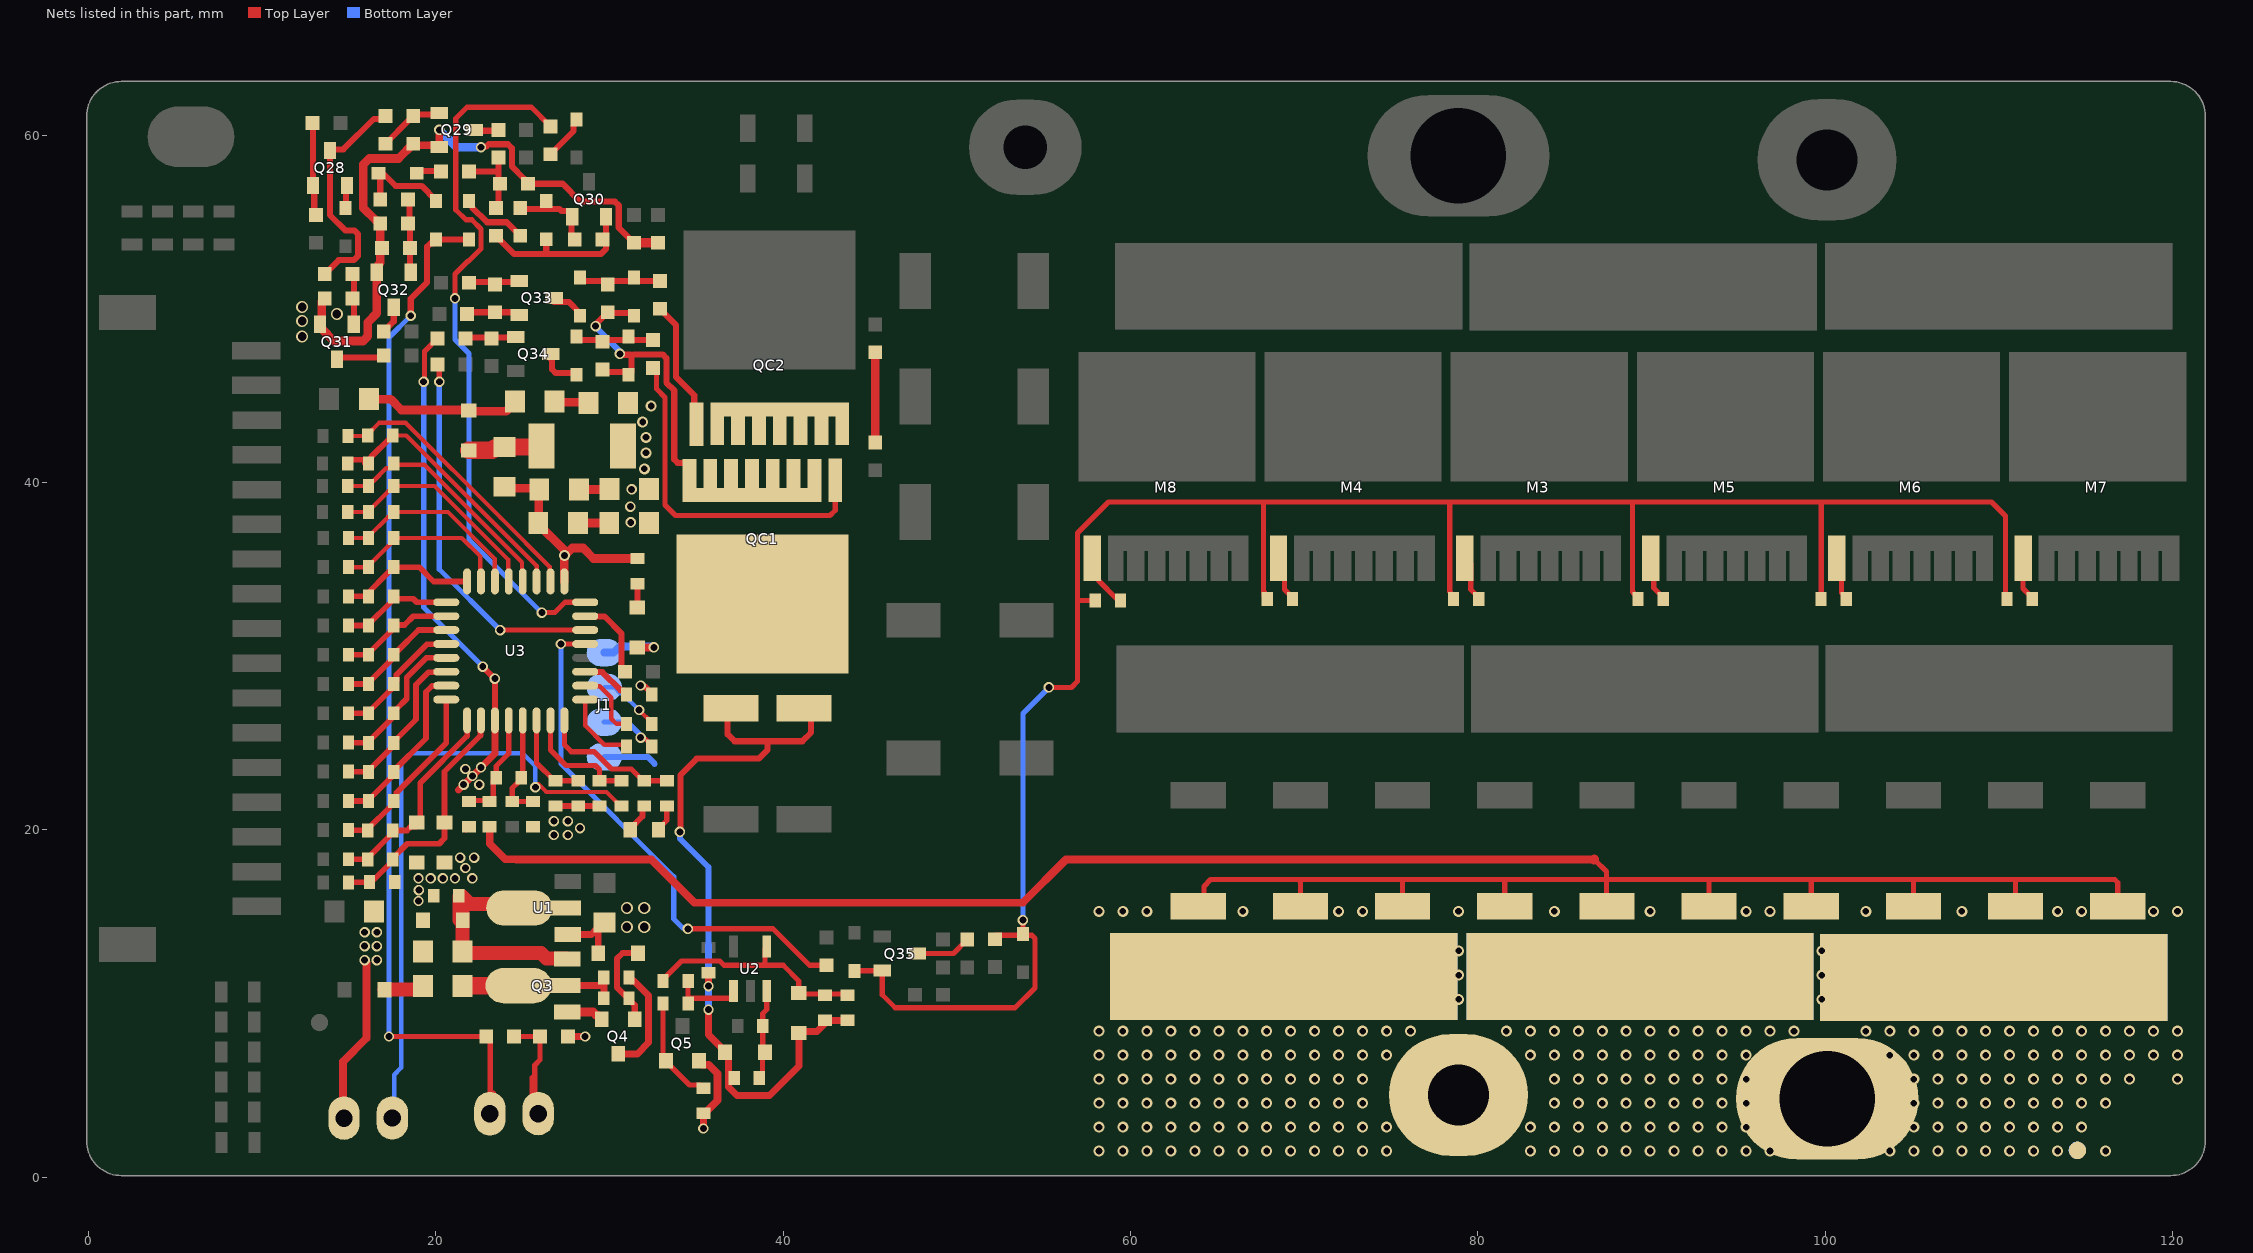
[diagram p0: the nets of this part, all layers, seen from the top]
# Altium PCB MISC86327.PcbDoc (part 2 of 2)
Units mm, origin at the board's own origin, x right, y up, seen from the top; angles counter-clockwise.
Board outline 122 x 63 mm, 2 copper layers (Top Layer, Bottom Layer); 198 components, 117 nets, 551 pads, 998 vias.
Unrouted connection lines stored in the file: 65.

## Via types
v1: diameter 0.635, hole 0.381, Top Layer to Bottom Layer, tented both sides, 846 vias
v2: diameter 0.6, hole 0.4, Top Layer to Bottom Layer, tented both sides, 133 vias
v3: diameter 0.635, hole 0.4, Top Layer to Bottom Layer, tented both sides, 11 vias
v4: diameter 0.7, hole 0.5, Top Layer to Bottom Layer, tented both sides, 8 vias

## Nets (pads, with @x,y where several pads share a name; then routed paths per layer and width w, separated by ;. In a path a pad name is that pad's centre, name@x,y a point inside that pad or via, vN(x,y) a via of type N, cw(c..) or ccw(c..) an arc to the next point about the centre after c; other vN are vias at no path point) (continued)
GND: C2.2 C3.2 C4.2 C6.1 C11.2 C16.2 C25.2 C34.1 C35.1 C36.1 C37.2 C40.2 C41.2 C51.1 C52.1 C53.1 D7.A D8.A D10.A D19.A D20.A J1.4 pad.28@114.522,1.542 pad.29 pad.30@78.88,4.73 pad.30@100.11,4.51 pad.31@68.82,11.55 pad.31@89.33,11.55 pad.31@109.7,11.5 pad.32@68.82,11.55 pad.32@89.33,11.55 pad.32@109.7,11.5 Q5.E Q29.E Q31.E Q32.E R16.1 R76.2 R87.1 R93.1 R126.1 R130.1 R139.1 R140.2 R141.1 R150.2 RN1.1 RN2.1 RN3.1 RN4.1 RN5.1 RN6.1 RN7.1 RN8.1 RN9.1 RN10.1 RT1.2 RT2.2 U1.1 U3.19 | length 233.8
  Top Layer w0.3: v2(19.3,45.8) 19.35,45.85 19.35,46.8 19.35,47.55 R150.2@20.1,48.3 ; RN10.1@63.9,15.602 64.223,15.925 64.223,16.74 64.613,17.13 69.67,17.13 ; RN9.1@69.783,15.602 69.783,17.017 69.67,17.13 ; RN8.1@75.666,15.602 75.666,17.126 75.67,17.13 ; RN7.1@81.549,15.602 81.549,17.116 81.535,17.13 ; 86.69,18.3 87.4,17.59 87.4,17.13 ; RN6.1@87.432,15.602 87.4,15.634 87.4,17.13 ; RN5.1@93.315,15.602 93.315,17.085 93.27,17.13 ; RN4.1@99.198,15.602 99.198,17.092 99.16,17.13 ; RN3.1@105.081,15.602 105.081,17.079 105.03,17.13 ; RN2.1@110.964,15.602 110.964,17.017 110.851,17.13 ; RN1.1@116.847,15.602 116.847,16.954 116.671,17.13 110.851,17.13 ; 69.67,17.13 75.67,17.13 ; 75.67,17.13 81.535,17.13 ; 81.535,17.13 87.4,17.13 ; 87.4,17.13 93.27,17.13 ; 93.27,17.13 99.16,17.13 ; 99.16,17.13 105.03,17.13 ; 105.03,17.13 110.851,17.13
  Top Layer w0.35: v2(22.6,59.3) 22.648,59.348 22.918,59.348 23.045,59.475 24.155,59.475 24.375,59.255 24.375,58.195 25.075,57.495 25.075,57.425 C52.1@25.3,57.2 27.3,57.2 28.325,56.175 30.305,56.175 30.53,55.95 30.53,54.67 R126.1@31.4,53.8 ; v2(22.7,29.4) v2(23.4,28.7) U3.19@23.4,26.3 ; R76.2@26.9,21.375 C35.1@28.2,21.375 C36.1@29.43,21.375 ; RT1.2@31.187,20 31.187,20.063 31.888,20.764 31.888,21.263 C34.1@32,21.375 ; v2(31.788,28.309) 31.836,28.262 32.038,28.262 32.425,27.875 C25.2@32.425,27.8
  Top Layer w0.4: 21.3,22.3 23.4,24.4 U3.19@23.4,26.3 ; U1.1@27.597,13.976 28.959,13.976 C2.2@29.265,14.282 ; R140.2@27.6,8.1 v2(28.6,8.1) ; D8.A@29.35,12.9 29.35,14.307 C2.2@29.7,14.657 ; v2(35.4,2.8) R16.1@35.4,3.675
  Top Layer w0.45: RT2.2@14.712,3.897 14.659,3.95 14.659,6.659 16,8 16,12.359 15.9,12.459 v2(15.9,12.5) ; R130.1@18.7,59.5 18.787,59.412 20.113,59.412 Q29.E@20.2,59.325 v2(20.2,60.3) ; D20.A@20.5,18.111 D20.A@20.55,18.111 ; C40.2@21.725,20.075 21.825,20.175 C40.2@21.9,20.175 ; R93.1@23.012,20.175 23.1,20.087 23.1,19.2 24,18.3 24.616,18.3 24.631,18.285 32.411,18.285 34.896,15.8 53.8,15.8 56.285,18.285 86.675,18.285 ; Q5.E@35.15,6.7 35.15,6.65 35.325,6.475 35.705,6.475 36.225,5.955 36.225,4.425 35.475,3.675 R16.1@35.4,3.675
  Top Layer w0.5: R141.1@13.6,50.6 13.425,50.425 13.425,48.85 14.125,48.15 15.811,48.15 16.075,48.414 16.075,49.211 16.6,49.736 Q32.E@16.6,52.1 16.675,52.175 16.675,52.522 16.8,52.647 R139.1@16.8,54.9 16.65,55.05 16.578,55.05 15.825,55.803 15.825,58.311 16.164,58.65 17.85,58.65 R130.1@18.7,59.5
  Top Layer w0.55: R126.1@31.4,53.8 C51.1@32.8,53.8 ; 86.675,18.285 86.69,18.3
  Bottom Layer w0.254: pad.31@67.163,12.907 pad.31@68.52,11.55
  Bottom Layer w0.3: v2(19.3,45.8) 19.3,32.8 v2(22.7,29.4) v2(23.4,28.7)
  Bottom Layer w0.35: J1.4@29.7,24.2 32.2,24.2 32.6,23.8
  Bottom Layer w0.5: v2(20.2,60.3) 21.2,59.3 v2(22.6,59.3)
  other v1: 58.182,1.502 59.562,1.502 60.942,1.502 62.322,1.502 63.702,1.502 65.082,1.502 66.462,1.502 67.842,1.502 69.222,1.502 70.602,1.502 71.982,1.502 73.362,1.502 74.742,1.502 83.022,1.502 84.402,1.502 85.782,1.502 87.162,1.502 88.542,1.502 89.922,1.502 91.302,1.502 92.682,1.502 94.062,1.502 95.442,1.502 96.822,1.502 103.722,1.502 105.102,1.502 106.482,1.502 107.862,1.502 109.242,1.502 110.622,1.502 112.002,1.502 113.382,1.502 116.142,1.502 58.182,2.882 59.562,2.882 60.942,2.882 62.322,2.882 63.702,2.882 65.082,2.882 66.462,2.882 67.842,2.882 69.222,2.882 70.602,2.882 71.982,2.882 73.362,2.882 74.742,2.882 83.022,2.882 84.402,2.882 85.782,2.882 87.162,2.882 88.542,2.882 89.922,2.882 91.302,2.882 92.682,2.882 94.062,2.882 95.442,2.882 105.102,2.882 106.482,2.882 107.862,2.882 109.242,2.882 110.622,2.882 112.002,2.882 113.382,2.882 114.762,2.882 58.182,4.262 59.562,4.262 60.942,4.262 62.322,4.262 63.702,4.262 65.082,4.262 66.462,4.262 67.842,4.262 69.222,4.262 70.602,4.262 71.982,4.262 73.362,4.262 84.402,4.262 85.782,4.262 87.162,4.262 88.542,4.262 89.922,4.262 91.302,4.262 92.682,4.262 94.062,4.262 95.442,4.262 105.102,4.262 106.482,4.262 107.862,4.262 109.242,4.262 110.622,4.262 112.002,4.262 113.382,4.262 114.762,4.262 116.142,4.262 58.182,5.642 59.562,5.642 60.942,5.642 62.322,5.642 63.702,5.642 65.082,5.642 66.462,5.642 67.842,5.642 69.222,5.642 70.602,5.642 71.982,5.642 73.362,5.642 84.402,5.642 85.782,5.642 87.162,5.642 88.542,5.642 89.922,5.642 91.302,5.642 92.682,5.642 94.062,5.642 95.442,5.642 105.102,5.642 106.482,5.642 107.862,5.642 109.242,5.642 110.622,5.642 112.002,5.642 113.382,5.642 114.762,5.642 116.142,5.642 117.522,5.642 120.282,5.642 58.182,7.022 59.562,7.022 60.942,7.022 62.322,7.022 63.702,7.022 65.082,7.022 66.462,7.022 67.842,7.022 69.222,7.022 70.602,7.022 71.982,7.022 73.362,7.022 74.742,7.022 83.022,7.022 84.402,7.022 85.782,7.022 87.162,7.022 88.542,7.022 89.922,7.022 91.302,7.022 92.682,7.022 94.062,7.022 95.442,7.022 103.722,7.022 105.102,7.022 106.482,7.022 107.862,7.022 109.242,7.022 110.622,7.022 112.002,7.022 113.382,7.022 114.762,7.022 116.142,7.022 117.522,7.022 118.902,7.022 120.282,7.022 58.182,8.402 59.562,8.402 60.942,8.402 62.322,8.402 63.702,8.402 65.082,8.402 66.462,8.402 67.842,8.402 69.222,8.402 70.602,8.402 71.982,8.402 73.362,8.402 74.742,8.402 76.122,8.402 81.642,8.402 83.022,8.402 84.402,8.402 85.782,8.402 87.162,8.402 88.542,8.402 89.922,8.402 91.302,8.402 92.682,8.402 94.062,8.402 95.442,8.402 96.822,8.402 98.202,8.402 102.342,8.402 103.722,8.402 105.102,8.402 106.482,8.402 107.862,8.402 109.242,8.402 110.622,8.402 112.002,8.402 113.382,8.402 114.762,8.402 116.142,8.402 117.522,8.402 118.902,8.402 120.282,8.402 78.89,10.233 99.802,10.232 78.89,11.633 99.802,11.632 78.89,13.033 99.802,13.032 58.182,15.302 59.562,15.302 60.942,15.302 66.462,15.302 71.982,15.302 73.362,15.302 78.882,15.302 84.402,15.302 89.922,15.302 95.442,15.302 96.822,15.302 102.342,15.302 107.862,15.302 113.382,15.302 114.762,15.302 118.902,15.302 120.282,15.302 32.01,40.78 32.1,41.7 32.1,42.6 31.91,43.48 32.4,44.4
  other v2: 16.6,12.5 15.9,13.3 16.6,13.3 15.9,14.1 16.6,14.1 19,15.9 19.024,16.521 19,17.2 19.7,17.2 20.4,17.2 21.1,17.2 22.1,17.2 21.7,17.8 21.4,18.4 22.2,18.4 26.8,19.7 27.6,19.7 28.3,20.1 26.8,20.5 27.6,20.5 21.6,22.6 22.5,22.6 22.1,23.1 21.7,23.5 22.6,23.6 31.222,37.702 31.202,38.612 31.272,39.602
  other v4: 31,14.4 32,14.4 31,15.5 32,15.5 12.3,48.4 12.3,49.3 14.3,49.7 12.3,50.1
GND1: C7.2 C12.2 C13.2 D11.A D12.A QC1.3 R18.1 RN13.1 RN14.1 | length 44.6
  Top Layer w0.35: v2(34.052,19.885) 34.075,19.907 34.075,23.153 35.022,24.1 38.6,24.1 39.1,24.6 39.1,25.1 ; RN14.1@37,27 36.8,26.8 36.8,25.5 37.2,25.1 39.1,25.1 ; RN13.1@41.2,27 41.6,26.6 41.6,25.6 41.1,25.1 39.1,25.1
  Top Layer w0.4: v2(35.7,9.65) 35.7,8.2 36.65,7.25 D11.A@36.65,7.2 36.85,7 36.85,5.2 37.35,4.7 39.2,4.7 40.9,6.4 D12.A@40.9,8.303 40.987,8.39 41.95,8.39 42.587,9.028 R18.1@43.7,9.028 ; v2(35.7,11) C7.2@35.7,11.775 ; C12.2@36.9,5.7 C12.2@37.175,5.7
  Bottom Layer w0.35: v2(34.052,19.885) 34.048,19.88 34.048,19.498 35.7,17.846 35.7,13.4
  Bottom Layer w0.4: v2(35.7,9.65) v2(35.7,11) 35.7,13.4
NetC3_1: C3.1 C4.1 D7.K Q3.E U1.2 | length 14.3
  Top Layer w0.8: D7.K@21.368,14.8 C4.1@21.368,16.157 ; C4.1@21.5,16.2 C4.1@21.543,16.157 ; U1.2@24.803,15.5 24.567,15.736 21.964,15.736 C4.1@21.543,16.157 ; Q3.E@27.556,12.552 27.524,12.584 26.381,12.584 26.064,12.9 21.643,12.9 C3.1@21.543,13 C4.1@21.543,16.157
NetC5_1: C5.1 C6.2 | length 2
  Top Layer w0.5: C5.1@26.833,44.66 26.873,44.62 28.747,44.62 C6.2@28.787,44.58
NetC5_2: C5.2 D9.A R12.2 | length 9
  Top Layer w0.5: R12.2@16.143,44.8 17.4,44.8 18.025,44.175 21.825,44.175 21.9,44.1 24.051,44.1 24.547,44.596 C5.2@24.547,44.66
NetC10_2: C10.2 C11.1 | length 1.8
  Top Layer w0.5: C10.2@28.238,39.582 28.253,39.597 29.977,39.597 C11.1@29.992,39.612
NetC12_1: C12.1 D11.K R17.1 U2.3 | length 5
  Top Layer w0.3: C12.1@38.625,5.7 38.8,5.875 38.8,7.05 D11.K@38.95,7.2 ; D11.K@38.825,7.2 R17.1@38.825,8.7 38.825,9.425 39.053,9.653 U2.3@39.053,10.5
NetC13_1: C13.1 D12.K R13.1 R18.2 U2.4 | length 13.3
  Top Layer w0.3: R13.1@33.075,11.375 34.15,12.45 36.35,12.45 36.6,12.2 38.8,12.2 ; U2.4@38.949,13.166 38.949,12.348 38.8,12.2 ; R18.2@43.7,10.478 43.637,10.54 40.962,10.54 D12.K@40.9,10.603 40.9,11.3 40,12.2 38.8,12.2
NetC15_2: C15.2 C16.1 | length 1.8
  Top Layer w0.5: C15.2@28.182,37.662 28.187,37.667 29.977,37.667 C16.1@29.982,37.672
NetC34_2: C34.2 R78.1 U3.24 | length 8.2
  Top Layer w0.3: U3.24@27.4,26.3 27.4,24.9 27.8,24.5 29.107,24.5 30.107,23.5 31.25,23.5 31.925,22.825 C34.2@32,22.825 R78.1@33.3,22.825
NetC35_2: C35.2 R76.1 U3.22 | length 5.3
  Top Layer w0.3: U3.22@25.8,26.3 25.8,23.85 26.825,22.825 R76.1@26.9,22.825 C35.2@28.2,22.825
NetC36_2: C36.2 R77.1 U3.23 | length 6.9
  Top Layer w0.3: U3.23@26.6,26.3 26.6,24.6 27.5,23.7 29.2,23.7 29.43,23.47 C36.2@29.43,22.825 R77.1@30.7,22.825
NetC39_1: C39.1 C41.1 R95.2 U3.21 | length 6.1
  Top Layer w0.3: C39.1@24.925,23 24.925,22.925 24.75,22.75 24.4,22.4 R95.2@24.4,21.625 C41.1@25.6,21.625 ; C39.1@25,23 U3.21@25,26.3
NetC39_2: C39.2 C40.1 R93.2 U3.20 | length 6.5
  Top Layer w0.3: C40.1@21.692,21.679 R93.2@23.066,21.679 ; R93.2@23.1,21.625 23.125,21.625 23.3,21.8 23.3,22.825 C39.2@23.475,23 ; C39.2@23.474,22.999 23.474,23.674 24.2,24.4 U3.20@24.2,26.3
NetC49_1: C49.1 C50.2 | length 5.2
  Top Layer w0.5: C50.2@45.3,42.3 C49.1@45.3,47.5
NetC53_2: C53.2 Q32.B R138.1 R139.2 | length 4.2
  Top Layer w0.35: R138.1@18.487,56.212 18.487,54.987 R139.2@18.4,54.9 18.5,54.8 Q32.B@18.5,52.071
NetD6_K: D6.K R9.2 | length 2.3
  Top Layer w0.8: D6.K@17.05,10.8 19.086,10.8 19.257,10.971 R9.2@19.257,11
NetD8_K: D8.K Q4.B R11.2 | length 5.3
  Top Layer w0.35: Q4.B@31.45,9.1 31.45,9.9 30.425,10.925 30.425,12.578 30.747,12.9 D8.K@31.65,12.9
NetD9_K: D9.K D10.K R20.2 | length 4.3
  Top Layer w1: D9.K@21.9,41.85 23.254,41.85 23.371,41.967 23.87,41.967 R20.2@23.942,42.038 25.958,42.038 D10.K@26.092,42.172
NetD13_A: D13.A J1.1 | length 3.8
  Top Layer w0.45: D13.A@31.6,30.5 v2(32.55,30.5)
  Bottom Layer w0.45: J1.1@29.7,30.2 30.233,30.2 30.583,30.55 v2@32.409,30.55
NetD13_K: D13.K R29.1 | length 1.4
  Top Layer w0.35: D13.K@31.6,32.8 R29.1@31.6,34.175
NetD35_A: D35.A Q28.E | length 1.3
  Top Layer w0.35: D35.A@14.8,55.8 14.837,55.838 14.837,57.062 Q28.E@14.875,57.1
NetD36_A: D36.A Q30.B R131.1 R133.1 | length 4.6
  Top Layer w0.35: R133.1@24.857,55.806 24.907,55.756 27.107,55.756 27.238,55.625 27.675,55.625 27.85,55.45 Q30.B@27.85,55.3 ; Q30.B@27.8,55.3 27.8,54.3 R131.1@28,54.1
NetD36_K: D36.K Q30.E R129.1 R131.2 | length 9.7
  Top Layer w0.35: R129.1@23.457,54.206 24.513,53.15 29.495,53.15 29.8,53.455 29.8,55.25 29.75,55.3 Q30.E@29.75,55.5 ; 26.357,53.306 D36.K@26.357,54.006
NetD37_A: D37.A R132.2 | length 1.4
  Top Layer w0.35: D37.A@18.9,57.9 18.925,57.925 R132.2@20.275,57.925
NetD37_K: D37.K D39.A R138.2 | length 5.5
  Top Layer w0.35: R138.2@16.8,56.3 16.8,57.879 16.871,57.879 17.675,57.075 19.175,57.075 20,56.25 D39.A@20,56.2
NetD38_A: D38.A R133.2 | length 3.9
  Top Layer w0.35: D38.A@21.9,56.2 22.075,56.025 22.075,55.858 22.951,54.981 24.082,54.981 R133.2@24.857,54.206
NetD38_K: D38.K D39.K R137.1 S1.1 | length 59.5
  Top Layer w0.3: v2(17.3,8.1) R137.1@22.9,8.1 23.128,7.872 23.128,4.327 23.3,4.154 S1.1@23.3,4.846
  Top Layer w0.35: v2(18.554,49.6) 18.554,50.579 19.5,51.525 19.5,53.57 19.705,53.775 19.825,53.775 20,53.95 D39.K@20,54 D38.K@22,54
  Bottom Layer w0.3: v2(17.3,8.1) 17.3,48.346 v2(18.554,49.6)
NetD40_A: D40.A R142.1 | length 2.4
  Top Layer w0.35: R142.1@26.6,58.9 27.925,60.225 27.925,60.525 D40.A@28.1,60.7
NetD41_A: D41.A Q33.C | length 1.8
  Top Layer w0.35: Q33.C@26.816,50.4 27.65,50.4 28.3,49.75 D41.A@28.3,49.7
NetD41_K: D41.K D44.K R152.1 RC1.1 | length 4.7
  Top Layer w0.35: D41.K@28.25,51.6 29.6,51.6 31.3,51.6 RC1.1@32.9,51.6
NetD42_A: D42.A Q34.C | length 2.3
  Top Layer w0.35: Q34.C@26.516,47.2 26.52,47.2 26.695,47.025 26.695,46.505 26.9,46.3 D42.A@28.1,46.3
NetD42_K: D42.K D45.K R153.2 RC2.2 | length 4.8
  Top Layer w0.35: D42.K@28.1,48.5 28.1,48.45 28.35,48.2 29.7,48.2 31.2,48.2 RC2.2@32.7,48.2
NetD43_K: D43.K DZ1.K Q35.E R110.1 R111.1 R114.1 R118.1 R121.1 R122.1 R156.2 | length 125.9
  Top Layer w0.3: D43.K@44.1,11.875 44.113,11.887 45.688,11.887 Q35.E@45.7,11.9 45.7,10.5 46.45,9.75 53.35,9.75 54.5,10.9 54.5,13.749 54.324,13.925 53.8,13.925 52.25,13.925 R156.2@52,13.675 ; DZ1.K@53.8,14 v2(53.8,14.8) ; v2(55.3,28.2) 56.6,28.2 56.95,28.55 56.95,33.2 ; R122.1@57.975,33.2 56.95,33.2 ; R111.1@67.875,33.3 67.7,33.475 67.7,33.688 67.662,33.726 67.662,38.87 ; R110.1@78.6,33.3 78.425,33.475 78.425,33.681 78.381,33.726 78.381,38.87 ; R114.1@89.215,33.3 89.215,33.375 88.9,33.69 88.9,38.87 ; R118.1@99.77,33.621 99.77,38.85 99.79,38.87 ; R121.1@110.377,33.28 110.377,38.063 109.57,38.87 99.79,38.87 ; 56.95,33.2 56.95,37.087 58.733,38.87 67.662,38.87 ; 67.662,38.87 78.381,38.87 ; 78.381,38.87 88.9,38.87 ; 88.9,38.87 99.79,38.87
  Bottom Layer w0.3: v2(53.8,14.8) 53.8,26.7 v2(55.3,28.2)
NetD44_A: D44.A D45.A QC1.2 QC2.2 R152.2 R153.1 | length 17.7
  Top Layer w0.35: v2(29.2,49) 29.248,49.048 29.248,49.148 R152.2@29.85,49.75 ; R153.1@29.7,46.5 29.85,46.35 31.15,46.35 D45.A@31.2,46.3 ; R152.2@29.75,49.75 31.25,49.75 D44.A@31.3,49.7 ; v2(30.6,47.4) 30.648,47.352 31.198,47.352 31.275,47.275 31.275,46.375 D45.A@31.1,46.2 ; 31.375,47.375 33.055,47.375 33.275,47.155 33.275,46.045 33.273,46.042 33.273,45.752 33.725,45.3 33.725,41.327 33.93,41.122 34.375,41.122 34.6,40.897 QC1.2@34.6,40.5
  Bottom Layer w0.35: v2(29.2,49) 29.2,48.95 30.7,47.45 v2@30.7,47.4
NetJ1_2: J1.2 R38.1 | length 3.6
  Top Layer w0.25: v2(31.7,26.9) 32.425,26.175 R38.1@32.425,26.1
  Bottom Layer w0.25: J1.2@29.7,28.2 30.287,28.2 30.623,27.864 30.736,27.864 v2(31.7,26.9)
NetJ1_3: J1.3 R36.1 | length 3.4
  Top Layer w0.25: v2(31.788,25.309) 31.855,25.242 32.058,25.242 32.425,24.875 R36.1@32.425,24.8
  Bottom Layer w0.3: J1.3@29.7,26.2 31.05,26.2 31.73,25.52 31.73,25.367 v2(31.788,25.309)
NetM3_G: M3.G R110.2 | length 2.7
  Top Layer w0.3: M3.G@79.237,35.637 79.587,35.287 79.587,33.838 80.05,33.375 R110.2@80.05,33.3
NetM4_G: M4.G R111.2 | length 2.7
  Top Layer w0.3: M4.G@68.518,35.637 68.868,35.287 68.868,33.832 69.325,33.375 R111.2@69.325,33.3
NetM5_G: M5.G R114.2 | length 2.6
  Top Layer w0.3: M5.G@90.122,35.662 90.122,33.931 R114.2@90.753,33.3
NetM6_G: M6.G R118.2 | length 2.5
  Top Layer w0.3: M6.G@100.932,35.637 100.932,33.651 R118.2@101.293,33.29
NetM7_G: M7.G R121.2 | length 2.6
  Top Layer w0.3: M7.G@111.392,35.653 111.392,33.891 R121.2@112.003,33.28
NetM8_G: M8.G R122.2 | length 3
  Top Layer w0.3: M8.G@57.8,35.637 58.15,35.287 58.15,34.35 R122.2@59.225,33.275
NetQ3_B: Q3.B Q4.E | length 2.2
  Top Layer w0.5: Q3.B@27.556,9.504 29.068,9.504 29.272,9.3 29.4,9.3 29.55,9.15 Q4.E@29.55,9.1
NetQ3_C: Q3.C R9.1 R10.1 R11.1 | length 7.1
  Top Layer w0.4: Q3.C@27.048,11.028 29.597,11.028 29.675,10.95 ; R11.1@29.675,10.3 29.675,10.95 ; R10.1@29.675,11.5 29.675,10.95
  Top Layer w1: R9.1@21.543,11 21.557,11.014 24.748,11.014 Q3.C@24.762,11.028
NetQ4_C: Q4.C R10.2 | length 6.3
  Top Layer w0.4: Q4.C@30.5,7.1 31.6,7.1 32.25,7.75 32.25,10.466 31.416,11.3 31.25,11.3 31.125,11.425 R10.2@31.125,11.5
NetQ5_B: Q5.B R15.2 R16.2 | length 6.1
  Top Layer w0.3: Q5.B@33.075,6.7 R15.2@33.075,10 ; Q5.B@33.25,6.7 33.25,6.65 34.6,5.3 35.225,5.3 R16.2@35.4,5.125
NetQ28_B: Q28.B R123.1 R127.2 | length 5.1
  Top Layer w0.35: Q28.B@12.925,57.1 R127.2@12.925,60.425 ; Q28.B@13,57.1 13,55.5 R123.1@13.1,55.4
NetQ28_C: Q28.C R128.2 R136.2 | length 13.2
  Top Layer w0.35: R136.2@13.6,52 14.403,52.803 15.283,52.803 15.525,53.045 15.525,54.295 15.32,54.5 14.8,54.5 13.9,55.4 Q28.C@13.9,59.179 ; Q28.C@14.2,59.179 14.679,59.179 16.429,60.929 16.929,60.929 R128.2@17.1,61.1
NetQ29_B: Q29.B R128.1 R130.2 | length 3.8
  Top Layer w0.35: R128.1@17.1,59.5 18.475,60.875 R130.2@18.7,61.1 18.787,61.187 20.112,61.187 Q29.B@20.2,61.275
NetQ29_C: Q29.C R124.1 | length 1.5
  Top Layer w0.35: Q29.C@22.216,60.3 22.266,60.25 23.65,60.25 R124.1@23.7,60.2
NetQ31_B: Q31.B R136.1 R141.2 | length 3.1
  Top Layer w0.35: R136.1@15.285,52.163 15.285,50.6 15.285,49.19 Q31.B@15.375,49.1
NetQ31_C: Q31.C R134.1 | length 2.8
  Top Layer w0.35: Q31.C@14.3,47.084 14.408,47.192 16.892,47.192 R134.1@17,47.3
NetQ32_C: Q32.C R135.1 | length 1.6
  Top Layer w0.35: R135.1@17,48.7 17.575,49.275 Q32.C@17.575,50.084
NetQ33_B: Q33.B R145.1 R149.2 | length 2.9
  Top Layer w0.35: R149.2@21.9,51.5 21.95,51.55 24.75,51.55 Q33.B@24.8,51.6
NetQ33_E: Q33.E R143.1 R145.2 | length 3.1
  Top Layer w0.35: R143.1@21.8,49.7 21.9,49.8 24.65,49.8 Q33.E@24.8,49.65
NetQ34_B: Q34.B R144.1 R150.1 | length 2.9
  Top Layer w0.35: R150.1@21.7,48.3 21.737,48.337 24.562,48.337 Q34.B@24.6,48.375
NetQ35_C: Q35.C R155.1 | length 3.2
  Top Layer w0.3: Q35.C@47.716,12.875 49.8,12.875 R155.1@50.6,13.675
NetQC1_1: QC1.1 RC2.1 | length 20
  Top Layer w0.3: RC2.1@32.7,46.6 32.7,45.4 33.2,44.9 33.2,38.7 33.8,38.1 42.7,38.1 43,38.4 QC1.1@43,40.138
NetQC2_1: QC2.1 RC1.2 | length 7.4
  Top Layer w0.35: RC1.2@32.9,50 33.825,49.075 33.825,46.075 34.88,45.02 34.88,43.57 QC2.1@35,43.45
NetR13_2: R13.2 R15.1 U2.1 | length 4.3
  Top Layer w0.3: R15.1@34.525,10 R15.1@34.525,10.3 ; R13.2@34.525,11.3 R15.1@34.525,10.3 ; U2.1@37.148,10.73 37.148,10.404 37.044,10.3 R15.1@34.525,10.3
NetR77_2: R77.2 RT2.1 | length 35.4
  Top Layer w0.25: v2@25.909,22.632 26.365,22.175 29.825,22.175 30.625,21.375 R77.2@30.7,21.375
  Bottom Layer w0.25: RT2.1@17.492,3.407 17.6,3.515 17.6,5.9 18,6.3 18,23.834 18.566,24.4 25,24.4 25.727,23.673 v2(25.727,22.45)
NetR78_2: R78.2 RT1.1 | length 1.6
  Top Layer w0.3: RT1.1@32.813,20 32.813,20.063 33.3,20.551 R78.2@33.3,21.375
NetR137_2: R137.2 R140.1 S1.2 | length 7.2
  Top Layer w0.3: R137.2@24.5,8.1 R140.1@26,8.1 26,6.76 25.7,6.46 25.7,4.154 25.528,4.327 25.528,5.738
NetR142_2: R142.2 U3.32 | length 40.9
  Top Layer w0.3: v2(21.1,50.6) 21.1,51.995 21.855,52.75 21.895,52.75 22.6,53.455 22.6,54.59 22.065,55.125 21.73,55.125 21.15,55.705 21.15,60.95 21.8,61.6 25.5,61.6 R142.2@26.6,60.5 ; v2(26.1,32.5) 26.119,32.519 26.85,32.519 27.431,33.1 U3.32@28.6,33.1
  Bottom Layer w0.3: v2(21.1,50.6) 21.1,48.228 21.9,47.428 21.9,36.7 v2(26.1,32.5)
NetR146_2: R146.2 U3.31 | length 4.8
  Top Layer w0.35: U3.31@28.6,32.3 28.619,32.281 29.719,32.281 30.7,31.3 30.7,29.3 R146.2@30.9,29.1
NetR148_2: R148.2 U3.30 | length 21.7
  Top Layer w0.3: R148.2@20.1,46.8 20.2,46.7 v2(20.2,45.8) ; v2(23.7,31.5) U3.30@28.6,31.5
  Bottom Layer w0.3: v2(20.2,45.8) 20.2,35 v2(23.7,31.5)
NetR151_2: R151.2 U3.29 | length 29.8
  Top Layer w0.3: v2(27.2,30.7) U3.29@28.6,30.7 ; v2(34.512,14.3) 39.406,14.3 41.506,12.2 R151.2@42.5,12.2
  Bottom Layer w0.3: v2(27.2,30.7) 27.2,23.8 33.7,17.3 33.7,14.856 34.199,14.357 34.455,14.357 v2(34.512,14.3)
RXD_M: R36.2 U3.25 | length 4.4
  Top Layer w0.25: U3.25@28.6,27.5 28.6,26 29.7,24.9 30.875,24.9 R36.2@30.975,24.8
TXD_M: R38.2 U3.26 | length 4
  Top Layer w0.25: U3.26@28.6,28.3 28.637,28.263 29.437,28.263 30.1,27.6 30.1,26.4 30.4,26.1 R38.2@30.975,26.1
VBAT_M: C10.1 C15.1 R20.1 R29.2 U3.1 | length 12.1
  Top Layer w0.5: R20.1@24.027,39.667 25.867,39.667 C10.1@25.952,39.582 25.924,39.554 25.924,37.69 C15.1@25.896,37.662 ; C15.1@25.896,37.599 27.374,36.12 ; U3.1@27.4,34.3 v3(27.4,35.8) 27.437,35.8 27.862,36.225 28.481,36.225 29.081,35.625 R29.2@31.6,35.625
VC0: C33.2 C37.1 D20.K R84.2 U3.18 | length 14.3
  Top Layer w0.33: R84.2@14.964,16.97 14.979,16.985 16.16,16.985 C37.1@16.175,17 ; C37.1@16.244,16.944 17.525,18.225 C33.2@17.525,18.3 17.525,18.375 18.349,19.199 20.191,19.199 20.5,19.508 D20.K@20.5,20.411 20.5,23.35 22.577,25.427 22.577,26.277 U3.18@22.6,26.3
VC1: C32.2 C33.1 D19.K R80.2 U3.17 | length 12
  Top Layer w0.33: R80.2@14.964,18.302 C33.1@16.075,18.3 ; R80.2@14.964,18.302 R80.2@14.964,18.377 ; C33.1@16.075,18.3 16.075,18.375 17.365,19.665 C32.2@17.365,19.79 ; C32.2@17.525,19.966 18.345,19.966 18.555,20.176 18.865,20.176 19.1,20.411 19.1,22.7 21.8,25.4 U3.17@21.8,26.3
VC2: C31.2 C32.1 R75.2 U3.16 | length 10.4
  Top Layer w0.33: R75.2@14.964,19.984 14.973,19.975 16.066,19.975 C32.1@16.075,19.966 16.075,20.041 17.412,21.378 C31.2@17.412,21.563 ; C31.2@17.572,21.648 17.732,21.808 17.732,22.132 20.6,25 U3.16@20.6,27.5
VC3: C30.2 C31.1 R73.2 U3.15 | length 10.1
  Top Layer w0.33: R73.2@14.964,21.666 14.973,21.657 16.113,21.657 C31.1@16.122,21.648 16.122,21.723 17.412,23.013 17.412,23.171 C30.2@17.572,23.33 17.572,23.405 19.43,25.264 19.43,27.93 19.777,28.277 20.577,28.277 U3.15@20.6,28.3
VC4_M: C28.2 C30.1 R67.2 U3.14 | length 9.4
  Top Layer w0.33: R67.2@14.964,23.348 14.973,23.339 16.113,23.339 C30.1@16.122,23.33 16.122,23.405 17.412,24.696 17.412,24.915 18.855,26.358 18.855,28.355 19.577,29.077 20.577,29.077 U3.14@20.6,29.1
VC5: C26.2 C28.1 R61.2 U3.13 | length 8.9
  Top Layer w0.33: R61.2@14.964,25.03 14.979,25.015 16.107,25.015 C28.1@16.122,25 16.122,25.075 17.412,26.365 17.412,26.553 C26.2@17.572,26.713 ; C26.2@17.732,26.948 18.325,27.541 18.325,28.775 19.45,29.9 U3.13@20.6,29.9 21.192,29.9 U3.13@21.2,29.892
VC6: C24.2 C26.1 R55.2 U3.12 | length 7.6
  Top Layer w0.33: R55.2@14.964,26.713 C26.1@16.122,26.713 16.122,26.788 17.412,28.078 17.412,28.235 C24.2@17.572,28.395 17.732,28.555 17.732,28.932 19.477,30.677 20.577,30.677 U3.12@20.6,30.7
VC7: C23.2 C24.1 R52.2 U3.11 | length 6.8
  Top Layer w0.33: R52.2@15.052,28.395 C24.1@15.872,28.395 ; C24.1@16.122,28.395 16.122,28.47 17.412,29.76 17.412,29.992 17.732,30.312 17.807,30.312 18.995,31.5 U3.11@20.6,31.5
VC8: C22.2 C23.1 R46.2 U3.10 | length 6.4
  Top Layer w0.33: R46.2@15.052,30.077 C23.1@15.929,30.077 ; C23.1@16.122,30.077 16.122,30.152 17.412,31.442 17.412,31.599 C22.2@17.572,31.759 17.611,31.799 18.199,31.799 18.7,32.3 U3.10@20.6,32.3
VC9: C20.2 C22.1 R42.2 U3.9 | length 6.5
  Top Layer w0.33: R42.2@15.052,31.759 C22.1@16.052,31.759 ; C22.1@16.122,31.759 16.122,31.834 17.412,33.124 17.412,33.281 C20.2@17.572,33.441 17.713,33.3 18.7,33.3 18.9,33.1 U3.9@20.6,33.1
VC10: C19.2 C20.1 R37.2 U3.8 | length 8.1
  Top Layer w0.33: R37.2@15.052,33.441 C20.1@16.175,33.441 ; C20.1@15.916,33.468 17.337,34.889 17.412,34.889 17.572,35.048 C19.2@17.572,35.123 19.049,35.123 19.873,34.3 U3.8@21.8,34.3
VC11: C18.2 C19.1 R32.2 U3.7 | length 10.1
  Top Layer w0.25: R32.2@15.052,35.123 C19.1@16.297,35.123 ; C19.1@16.3,35.377 17.372,36.448 17.372,36.606 C18.2@17.572,36.806 21.494,36.806 22.563,35.737 22.563,34.337 U3.7@22.6,34.3
VC12: C17.2 C18.1 R28.2 U3.6 | length 11.6
  Top Layer w0.25: R28.2@14.964,36.806 C18.1@16.122,36.806 16.122,36.881 17.266,38.025 17.372,38.025 17.572,38.225 C17.2@17.572,38.3 20.7,38.3 23.4,35.6 U3.6@23.4,34.3 ; C17.2@17.518,38.354 C17.2@17.572,38.354
VC13: C14.2 C17.1 R25.2 U3.5 | length 12.9
  Top Layer w0.25: R25.2@14.925,38.3 C17.1@16.122,38.3 16.122,38.375 16.322,38.575 16.347,38.575 17.297,39.525 17.372,39.525 C14.2@17.572,39.725 ; C14.2@17.572,39.8 19.927,39.8 24.162,35.565 24.162,34.338 U3.5@24.2,34.3
VC14: C9.2 C14.1 R23.2 U3.4 | length 14.3
  Top Layer w0.25: R23.2@14.925,39.8 C14.1@16.122,39.8 ; R23.2@15.052,39.97 R23.2@15.062,39.96 ; C9.2@17.57,41.225 17.77,41.025 19.339,41.025 24.963,35.4 24.963,34.337 U3.4@25,34.3
  Top Layer w0.254: C14.1@16.122,39.8 16.122,39.875 16.32,40.073 16.395,40.073 17.149,40.827 17.372,40.827 17.57,41.025 C9.2@17.57,41.225
VC15: C8.2 C9.1 R21.2 U3.3 | length 15.8
  Top Layer w0.25: C8.2@17.525,42.7 18.3,42.7 25.8,35.2 U3.3@25.8,34.3
  Top Layer w0.33: R21.2@14.925,41.3 C9.1@16.12,41.3 ; C9.1@15.912,41.1 C9.1@16.238,41.1 ; C9.1@16.12,41.1 16.12,41.32 16.265,41.32 16.28,41.335 16.28,41.48 C8.2@17.311,42.511
VC16: C8.1 R19.2 U3.2 | length 16.3
  Top Layer w0.254: R19.2@14.947,42.675 16.05,42.675 C8.1@16.075,42.7 16.075,42.775 16.727,43.427 18.273,43.427 23.748,37.952 26.563,35.137 26.563,34.337 U3.2@26.6,34.3
VCC1: C52.2 R125.2 R129.2 R132.1 | length 4.3
  Top Layer w0.35: R132.1@22.1,57.9 23.6,57.9 ; R129.2@23.6,55.6 C52.2@23.6,57 ; C52.2@23.6,57.1 23.6,57.9 ; R125.2@23.7,58.5 23.6,58.4 23.6,57.9
VCC_M: C25.1 U3.27 | length 3
  Top Layer w0.35: U3.27@28.6,29.1 28.619,29.081 29.589,29.081 30.645,28.025 30.825,28.025 30.975,27.875 C25.1@30.975,27.8
pads on no net: J2.0

## Polygon pours and split planes (outlines as drawn)
BC16 on Top Layer "NONET_L02_P-001" (solid, remove dead copper, pour order 212): -0.3,55.6 0,55.3 8.5,55.3 8.7,55.1 8.7,47.7 9.6,46.8 11.1,46.8 11.6,47.3 11.6,62.8 11.1,63.3 0.3,63.3 -0.3,62.7
BC0 on Top Layer "NONET_L02_P-001" (solid, remove dead copper, pour order 213): 7.8,13.004 8.382,12.4 14.8,12.4 14.8,14.682 14.8,15.163 14.8,16.009 14.2,16.609 14.2,17.3 14.1,17.4 12.9,17.4 11.9,16.4 7.8,16.4
BC16 on Top Layer "NONET_L02_P-001" (solid, remove dead copper, pour order 240): 8.8,0.7 9,0.5 11.66,0.5 11.8,0.64 11.8,6.2 12.8,7.2 13.8,7.2 15.2,8.6 15.2,11.3 14.7,11.8 9.4,11.8 8.8,11.2
CHGD1 on Top Layer "NONET_L02_P-001" (solid, remove dead copper, pour order 219): 39.6,55.7 40.4,54.9 44,54.9 44.3,54.6 44.3,46.3 44.2,46.2 34.4,46.2 34.1,46.5 34.1,62.7 34.3,62.9 39.3,62.9 39.6,62.6
NetD44_A on Top Layer "NONET_L02_P-001" (solid, remove dead copper, pour order 209): 42.7,42 44.1,42 44.1,45.3 43.7,45.7 36,45.7 35.6,45.3 35.6,42 34.1,42 34.1,38.8 34.2,38.7 42.3,38.7 42.4,38.8 42.4,41.7
GND on Top Layer "NONET_L02_P-001" (solid, remove dead copper, pour order 107): 55.1,0.03 120.03,0.03 ccw(c120.03,1.9) 121.9,1.9 121.82,10.18 121.82,15.11 ccw(c120.605,15.115) 120.61,16.33 56.13,16.33 55.1,15.3
GND on Top Layer "NONET_L02_P-001" (solid, remove dead copper, pour order 238): 23.3,25.6 23.5,25.6 23.6,25.5 23.6,24.4 23,23.8 23,22.6 22.5,22.1 21.1,22.1 21,22.2 21,23.3
GND on Top Layer "NONET_L02_P-001" (solid, remove dead copper, pour order 227): 11.8,48.3 12.2,47.9 14,47.9 14.5,48.4 14.5,51.1 14.4,51.2 11.8,51.2
GND on Top Layer "NONET_L02_P-001" (solid, remove dead copper, pour order 228): 32.4,13.8 32.5,13.9 32.5,15.8 32.395,15.905 29.705,15.905 28.2,14.4 27.3,14.4 27.243,14.343 27.243,13.5 28.4,13.5 28.8,13.1 28.8,12.5 28.9,12.4 29.8,12.4 29.8,12.937 30.663,13.8
NetR77_2 on Top Layer "NONET_L02_P-001" (solid, remove dead copper, pour order 204): 16.25,6.3 16.25,-0.05 19.5,-0.05 19.5,6.3
GND on Top Layer "NONET_L02_P-001" (solid, remove dead copper, pour order 226): 26.5,21.7 29.7,21.7 29.9,21.5 29.9,21.05 30.29,20.66 31.6,20.66 31.6,19.4 25.3,19.4 25,19.7 25,20.5 25.2,20.7 25.95,20.7 26.5,21.25
C- on Top Layer "NONET_L02_P-001" (solid, remove dead copper, pour order 193): 40.3,56.3 40.9,55.7 46.531,55.7 48.11,54.12 51.1,54.12 51.276,53.924 51.276,43.526 51.901,42.9 56,42.9 56.2,43.1 56.2,53.32 58.05,55.17 58.05,63.09 58.01,63.05 51.976,63.05 51.926,63.1 40.3,63.1
GND on Top Layer "NONET_L02_P-001" (solid, remove dead copper, pour order 222): 32.3,45.2 32.8,44.7 32.8,40.8 32.989,40.611 33.002,38.85 33.002,36.933 32.769,36.7 31.1,36.7 30.9,36.9 30.9,40.31 30.478,40.733 29.9,40.733 29.9,44.9 30.2,45.2
VBAT_M on Top Layer "NONET_L02_P-001" (solid, remove dead copper, pour order 223): 28.916,35.3 28.716,35.5 26.732,35.5 23.027,39.205 23.027,40.387 26.713,40.387 27.1,40 27.1,36.9 27.3,36.7 29.3,36.7 29.6,36.4 31.85,36.4 32.2,36.05 32.2,35.3
GND on Top Layer "NONET_L02_P-001" (solid, remove dead copper, pour order 221): 21.2,20.6 21.3,20.7 22.3,20.7 22.5,20.5 22.5,17 22.4,16.9 20.3,16.9 20.1,16.7 20.1,15.7 19.867,15.467 19.867,12.086 15.614,12.086 15.5,12.2 15.5,16.2 15.6,16.3 16.75,16.3 16.9,16.45 16.9,17 17.461,17.561 18.225,17.561 18.225,18.425 18.5,18.7 20.7,18.7 21.2,19.2
NetR137_2 on Top Layer "NONET_L02_P-001" (solid, remove dead copper, pour order 203): 24.458,6.6 24.458,0.197 27.9,0.197 27.9,6.6
NetD38_K on Top Layer "NONET_L02_P-001" (solid, remove dead copper, pour order 202): 21.178,6.5 21.178,0.187 24.078,0.187 24.078,6.5
GND1 on Top Layer "NONET_L02_P-001" (solid, remove dead copper, pour order 208): 33.7,37.2 34,37.5 44.1,37.5 44.4,37.2 44.4,27 43.7,26.3 34.1,26.3 33.7,26.7
BC16 on Top Layer "NONET_L02_P-001" (solid, remove dead copper, pour order 207): 46.2,53.5 46.2,34.9 49.8,34.9 50.5,35.6 50.5,52.9 49.9,53.5
DSGD1 on Top Layer "NONET_L02_P-001" (solid, remove dead copper, pour order 106): 45,29.3 45.3,29 55.6,29 56.3,29.7 56.3,32.885 56.3,37.17 58.63,39.5 121.81,39.5 121.81,61.121 ccw(c119.861,61.121) 119.861,63.07 82.83,63.07 60.21,63.08 ccw(c60.306,62.984) 60.18,63.036 58.939,63.036 cw(c58.939,63.119) 58.88,63.06 58.88,56.037 58.88,55.027 56.9,53.047 56.9,43.1 56.1,42.3 52,42.3 51.2,41.5 51.2,35 50.601,34.401 45.001,34.401 45,34.4
NetC3_1 on Top Layer "NONET_L02_P-001" (solid, remove dead copper, pour order 211): 21.2,16.6 26.1,16.6 27.089,15.611 27.089,15.089 26.4,14.4 21.5,14.4 21.2,14.7
DG- on Top Layer "NONET_L01_P-001" (solid, remove dead copper, pour order 165): 42.74,21.24 ccw(c42.74,21.8) 43.3,21.8 43.3,24.67 cw(c45.84,24.67) 45.84,27.21 56.409,27.21 57.6,28.401 57.6,32.1 58.075,32.575 59.733,32.575 ccw(c59.68,32.84) 59.95,32.84 59.95,37.85 cw(c60.48,37.85) 60.48,38.38 66.9,38.38 cw(c66.9,37.72) 67.56,37.72 67.56,33.06 ccw(c68.03,33.06) 68.03,32.59 70.3,32.59 ccw(c70.3,32.86) 70.57,32.86 70.57,37.88 cw(c71.05,37.88) 71.05,38.36 77.7,38.36 cw(c77.7,38.02) 78.04,38.02 78.04,33.25 ccw(c78.7,33.25) 78.7,32.59 80.72,32.59 ccw(c80.72,32.84) 80.97,32.84 80.97,37.96 cw(c81.38,37.96) 81.38,38.37 88.14,38.37 cw(c88.14,37.99) 88.52,37.99 88.52,32.99 ccw(c88.93,32.99) 88.93,32.58 91.03,32.58 ccw(c91.03,32.94) 91.39,32.94 91.39,37.67 cw(c92.13,37.67) 92.13,38.41 98.79,38.41 cw(c98.79,38.26) 98.94,38.26 98.94,33.09 ccw(c99.6,33.09) 99.6,32.43 101.8,32.43 ccw(c101.8,32.74) 102.11,32.74 102.11,37.5 cw(c102.98,37.5) 102.98,38.37 109.18,38.37 cw(c109.18,37.85) 109.7,37.85 109.7,32.79 ccw(c110.06,32.79) 110.06,32.43 112.24,32.43 ccw(c112.24,32.79) 112.6,32.79 112.6,38.06 cw(c112.94,38.06) 112.94,38.4 120.88,38.4 cw(c120.88,37.7) 121.58,37.7 121.58,21.95 cw(c120.87,21.95) 120.87,21.24 62.6,21.24 ccw(c62.6,20.47) 61.83,20.47 61.83,20.46 cw(c61.15,20.46) 61.15,19.78 55.88,19.78 53,16.9 36,16.9 35.4,17.5 35.4,21.24
GND on Top Layer "NONET_L02_P-001" (solid, remove dead copper, pour order 205): 12.5,6.1 12.7,6.3 15.87,6.3 15.87,-0.06 12.5,-0.06
GND on Bottom Layer "NONET_L02_P-001" (solid, remove dead copper, pour order 239): 18.6,28 20.8,25.8 25.8,25.8 26.5,26.5 26.5,29 25.4,30.1 23.8,30.1 20.6,33.3 20.6,33.5 19.8,34.3 19.8,47.3 19.6,47.5 18.6,47.5
GND on Bottom Layer "NONET_L02_P-001" (solid, remove dead copper, pour order 229): 30.7,34 30.65,33.95 30.65,25.75 28.1,25.75 28.1,21.7 25.4,21.7 23,24.1 19.7,24.1 18.6,23 18.6,7.2 20.1,5.7 33,5.7 34.2,4.5 34.2,0.3 34.5,0 59.9,0 60.2,0.3 60.2,12.7 58.3,14.6 52.725,14.6 52.2,15.125 52.2,33.9 51.699,34.401 44.599,34.401 32.6,46.4 24.814,46.4 23.836,45.422 23.836,37.164 24.5,36.5 28.2,36.5
BC7 on Bottom Layer "BC7_L02_P217" (solid, remove dead copper, pour order 217): 6.695,30.325 11.005,30.325 11.105,30.225 11.105,28.895 11.085,28.875 6.705,28.875
BC8 on Bottom Layer "BC8_L02_P242" (solid, remove dead copper, pour order 242): 9.53,32.37 9.53,30.93 9.52,30.92 6.019,30.92 6.009,32.37
BC9 on Bottom Layer "BC9_L02_P241" (solid, remove dead copper, pour order 241): 9.53,34.37 9.53,32.93 9.52,32.92 6.019,32.92 6.009,34.37
BC16 on Bottom Layer "NONET_L02_P-001" (solid, remove dead copper, pour order 199): 5.4,47.7 5.4,53.2 4.75,53.85 0.65,53.85 -0.2,54.7 -0.2,60.4 0.7,61.3 18.275,61.3 18.6,60.975 18.6,58.3 19.9,57 37.9,57 40.6,54.3 54.7,54.3 55.9,53.1 55.9,36 55.1,35.2 45.2,35.2 29.3,51.1 12.1,51.1 11.4,50.4 11.4,48.1 12.1,47.4 14.3,47.4 15,46.7 15,7.2 13.4,5.6 13.4,0.4 9.9,0.4 9.8,0.5 9.8,43.3
GND on Bottom Layer "NONET_L02_P-001" (solid, remove dead copper, pour order 230): 15.2,10 16.9,10 16.95,10.05 16.95,42.15 16.9,42.2 16.9,50.6 16.7,50.8 12.2,50.8 11.8,50.4 11.8,48.3 12.2,47.9 14.8,47.9 15.2,47.5
BC11 on Bottom Layer "BC11_L02_P197" (solid, remove dead copper, pour order 197): 5.996,38.3 9.51,38.3 9.51,36.85 6.006,36.85
BC12 on Bottom Layer "BC12_L02_P196" (solid, remove dead copper, pour order 196): 5.982,40.325 9.43,40.325 9.53,40.225 9.53,38.895 9.51,38.875 5.992,38.875
BC13 on Bottom Layer "BC13_L02_P195" (solid, remove dead copper, pour order 195): 5.968,42.325 9.53,42.325 9.53,40.875 5.978,40.875
BC14 on Bottom Layer "BC14_L02_P194" (solid, remove dead copper, pour order 194): 5.954,44.325 8,44.325 8,42.875 5.964,42.875
GND on Bottom Layer "NONET_L02_P-001" (solid, remove dead copper, pour order 225): 19,61.1 19,58.3 20,57.3 29.6,57.3 25.8,61.1 19.9,61.1
DSGD1 on Bottom Layer "NONET_L02_P-001" (solid, remove dead copper, pour order 103): 60.18,63.036 58.939,63.036 cw(c58.939,63.119) 58.88,63.06 58.88,56.037 cw(c56.811,56.037) 58.274,54.574 ccw(c60.07,52.778) 57.53,52.778 57.53,40.6 ccw(c58.63,40.6) 58.63,39.5 121.81,39.5 121.81,61.121 ccw(c119.861,61.121) 119.861,63.07 82.83,63.07 60.21,63.08 ccw(c60.307,62.983)
C- on Bottom Layer "C-_L02_P104" (solid, remove dead copper, pour order 104): 57.156,54.8 ccw(c57.156,56.065) 58.05,55.17 58.05,63.05 57.76,63.3 40.1,63.3 40,63.2 34,63.2 34,57.6 34.2,57.4 38.5,57.4 41.1,54.8
BC10 on Bottom Layer "BC10_L02_P198" (solid, remove dead copper, pour order 198): 9.53,36.37 9.53,34.93 9.52,34.92 6.019,34.92 6.009,36.37
DG- on Bottom Layer "NONET_L02_P-001" (solid, remove dead copper, pour order 108): 94.819,38.41 106.805,38.41 111.61,38.41 111.62,38.4 121.6,38.4 122,38 122,19.8 121.4,19.2 57.6,19.2 57.4,19.4 57.4,37.3 58.51,38.41 75.567,38.41 90.785,38.41
GND on Bottom Layer "Bottom Layer-GND" (solid, remove dead copper, pour order 112): 55.314,15.514 56.1,16.333 121.82,16.267 121.82,10.18 121.9,1.9 cw(c120.03,1.9) 120.03,0.03 89.325,0.03 56.7,0.03 55.314,1.416

## Keep-outs
Keep-Out Layer:
  circle w0.1: c118.84,60.09 r1.05
  circle w0.1: c31.48,3.09 r1.05
  circle w0.1: c118.84,3.09 r1.05
  circle w0.1: c31.48,60.09 r1.05
  pour cut-out: 29.17,60.09 ccw(c31.47,60.09) 31.47,57.79 ccw(c31.47,60.09) 33.77,60.09 ccw(c31.47,60.09) 31.47,62.39 ccw(c31.47,60.09)
  pour cut-out: 116.6,60.09 ccw(c118.85,60.09) 118.85,57.84 ccw(c118.85,60.09) 121.1,60.09 ccw(c118.85,60.09) 118.85,62.34 ccw(c118.85,60.09)
  pour cut-out: 29.18,3.09 ccw(c31.48,3.09) 31.48,0.79 ccw(c31.48,3.09) 33.78,3.09 ccw(c31.48,3.09) 31.48,5.39 ccw(c31.48,3.09)
  pour cut-out: 116.53,3.09 ccw(c118.83,3.09) 118.83,0.79 ccw(c118.83,3.09) 121.13,3.09 ccw(c118.83,3.09) 118.83,5.39 ccw(c118.83,3.09)
  lines w0.05: 30.405,60.09 cw(c30.43,60.09) 30.455,60.09 cw(c30.43,60.09) 30.405,60.09
  lines w0.1: 4.456,-452.691 ccw(c4.456,-450.691) 6.456,-450.691 ; -0.11,2.09 ccw(c1.89,2.09) 1.89,0.09 ; -0.11,2.09 ccw(c1.89,2.09) 1.89,0.09 ; -0.11,2.09 -0.11,61.09 ; -0.11,2.09 -0.11,61.09 ; -0.11,61.09 cw(c1.89,61.09) 1.89,63.09 ; -0.11,61.09 cw(c1.89,61.09) 1.89,63.09 ; 1.89,0.09 119.89,0.09 ccw(c119.89,2.09) 121.89,2.09 ; 1.89,63.09 119.89,63.09 ; 119.89,63.09 cw(c119.89,61.09) 121.89,61.09 ; 119.89,63.09 cw(c119.89,61.09) 121.89,61.09 ; 121.89,2.09 121.89,61.09 ; 121.89,2.09 121.89,61.09 ; 121.89,2.09 121.89,61.09 ; 121.89,2.09 121.89,61.09

## Other copper
Top Layer:
  rectangle net BC8: 6.019,30.772 11.153,32.372
  rectangle net NetC3_1: 21.2,12.3 22.5,16.6
  rectangle net BC0: 7.8,14.8 11.125,16.4
  rectangle net BC1: 7.8,16.8 11.125,18.4
  rectangle net BC2: 7.8,18.8 11.125,20.4
  rectangle net BC3: 7.8,20.838 11.163,22.438
  rectangle net BC4: 7.8,22.8 11.125,24.4
  rectangle net BC5: 7.8,24.8 11.125,26.4
  rectangle net BC6: 7.32,26.8 11.125,28.4
  rectangle net BC7: 7.275,28.8 11.125,30.4
  rectangle net BC9: 6.019,32.81 11.135,34.41
  rectangle net BC10: 6.014,34.8 11.125,36.4
  rectangle net BC11: 5.9,36.8 11.125,38.4
  rectangle net BC12: 5.9,38.8 11.125,40.4
  rectangle net BC13: 5.9,40.8 11.125,42.4
  rectangle net BC14: 5.9,42.8 11.125,44.4
  rectangle net BC15: 6.2,44.8 11.1,46.4
  rectangle net BC16: 7.6,46.8 11.1,48.4

## Silkscreen, mask and mechanical layers (free items; w line width, h text height)
Mechanical 41:
  circle w0.006: c9.99,0.09 r0.003
  circle w0.006: c9.99,63.09 r0.003